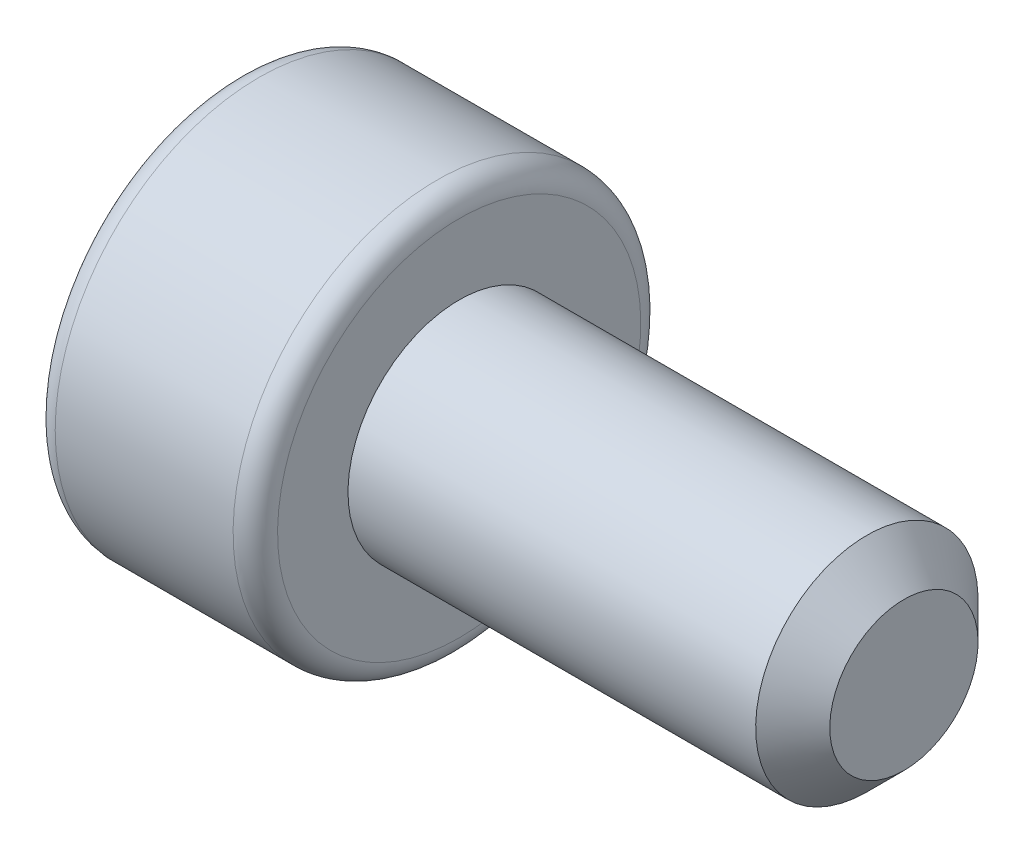
from build123d import *

# Parameters (mm, degrees)
CUT_EXTRUDE1_DEPTH = 1.3
FILLET1_R          = 0.3
CHAMFER1_SIZE      = 0.1
CHAMFER1_SIZE2     = 0.567128182
CHAMFER2_SIZE      = 0.5


with BuildPart() as part:
    # Sketch1 → Revolve1 (revolve)
    with BuildSketch(Plane.XY, mode=Mode.PRIVATE) as revolve1_sk:
        Polygon((0, 0), (0, 2.75), (3, 2.75), (3, 1.5), (9, 1.5), (9, 0), align=None)
    revolve(revolve1_sk.sketch.rotate(Axis((-4.709244637, 0, 0), (1, 0, 0)), 180), axis=Axis((-4.709244637, 0, 0), (1, 0, 0)))

    # Sketch4 → Cut-Extrude1 (cut)
    with BuildSketch(Plane.ZY):
        Polygon((-1.443375673, 0), (-0.721687836, -1.25), (0.721687836, -1.25), (1.443375673, 0), (0.721687836, 1.25), (-0.721687836, 1.25), align=None)
    extrude(amount=-CUT_EXTRUDE1_DEPTH, mode=Mode.SUBTRACT)

    # Fillet1
    fillet1_edges = [part.edges().sort_by_distance(p)[0] for p in [
        (3, 2.75, 0),
        (0, 2.75, 0),
    ]]
    fillet(fillet1_edges, radius=FILLET1_R)

    # Chamfer1
    chamfer1_edges = [part.edges().sort_by_distance(p)[0] for p in [
        (0, 0.625, -1.082531755),
        (0, -0.625, -1.082531755),
        (0, -1.25, 0),
        (0, -0.625, 1.082531755),
        (0, 0.625, 1.082531755),
        (0, 1.25, 0),
    ]]
    chamfer1_side = [part.faces().sort_by_distance(p)[0] for p in [
        (0, 2.380703535, 0),
    ]]
    chamfer(chamfer1_edges, length=CHAMFER1_SIZE, length2=CHAMFER1_SIZE2, reference=chamfer1_side[0])

    # Chamfer2
    chamfer2_edges = [part.edges().sort_by_distance(p)[0] for p in [
        (9, 1.5, 0),
    ]]
    chamfer(chamfer2_edges, length=CHAMFER2_SIZE)


solid = part.part
